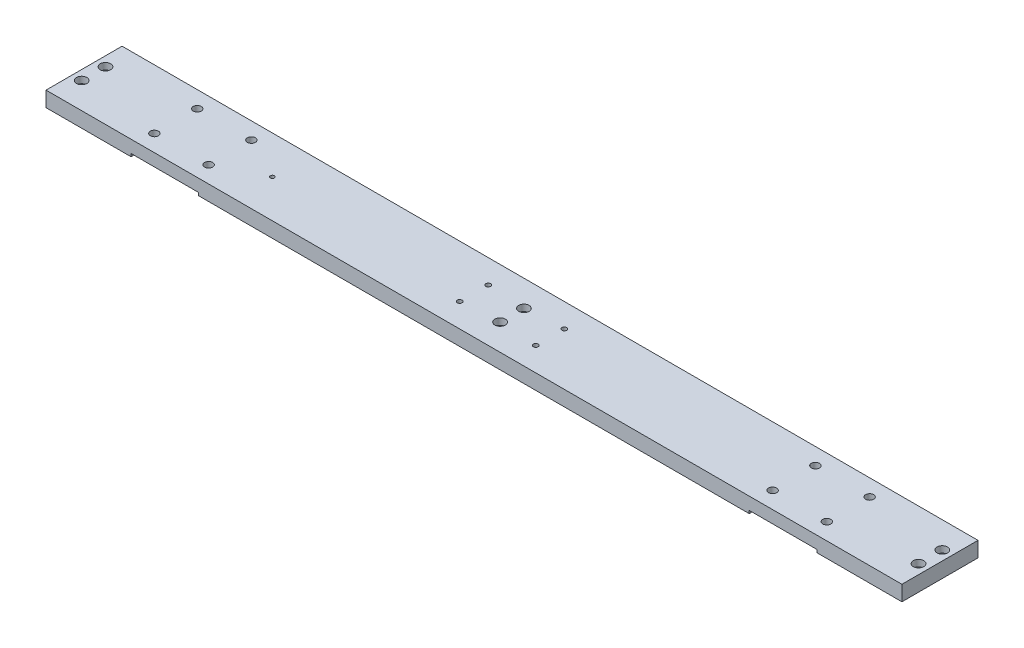
SolidWorks part; units mm, degrees
ref_plane "前视基准面" through (0, 0, 0) normal (0, 0, 1) x (1, 0, 0)
ref_plane "上视基准面" through (0, 0, 0) normal (0, 1, 0) x (1, 0, 0)
ref_plane "右视基准面" through (0, 0, 0) normal (1, 0, 0) x (0, 0, -1)
sketch "草图1" plane through (0, 0, 0) normal (0, 1, 0) x (1, 0, 0)
  line L1 (-450, 40) -> (450, 40)
  line L2 (-450, 40) -> (-450, -40)
  line L3 (-450, -40) -> (450, -40)
  line L4 (450, 40) -> (450, -40)
  line L5 (-450, 40) -> (450, -40) construction
  line L6 (-450, -40) -> (450, 40) construction
  point P0 (0, 0)
  dimension "D1" = 900
  dimension "D2" = 80
extrude "凸台-拉伸1" add sketch "草图1" along normal blind 16
sketch "草图2" plane through (0, 0, 0) normal (0, -1, 0) x (1, 0, 0)
  line L0 (-450, 40) -> (450, 40) construction
  line L1 (-360.549, 40) -> (-289.451, 40)
  line L2 (-360.549, 40) -> (-360.549, -40)
  line L3 (-360.549, -40) -> (-289.451, -40)
  line L4 (-289.451, 40) -> (-289.451, -40)
  line L5 (450, -40) -> (-450, -40) construction
  line L6 (0, 0) -> (0, 177.7451) construction
  line L7 (289.451, 40) -> (360.549, 40)
  line L8 (289.451, 40) -> (289.451, -40)
  line L9 (289.451, -40) -> (360.549, -40)
  line L10 (360.549, 40) -> (360.549, -40)
  dimension "D1" = 71.0981
  dimension "D2" = 650
extrude "切除-拉伸1" cut sketch "草图2" against normal blind 3
hole_wizard "Ø8.5 (8.5) 直径孔1" positions "草图3" profile "草图4" hole size "Ø8.5" standard "GB" end condition through all
sketch "草图3" plane through (0, 16, 0) normal (0, 1, 0) x (1, 0, 0)
  line L0 (0, 0) -> (-342.1751, 0) construction
  line L3 (-360.549, 40) -> (-289.451, 40) construction
  line L5 (-325, 40) -> (-325, 23.2164) construction
  point P0 (-353.5, 22.5)
  point P2 (-296.5, 22.5)
  point P4 (-353.5, -22.5)
  point P6 (-296.5, -22.5)
  dimension "D1" = 57
  dimension "D2" = 45
sketch "草图4" plane through (-353.5, 16, -22.5) normal (1, 0, 0) x (0, 0, 1)
  line L0 (0, 0) -> (0, 16)
  line L1 (0, 16) -> (4.25, 16)
  line L2 (4.25, 16) -> (4.25, 0)
  line L5 (4.25, 0) -> (0, 0)
  line L11 (0, -6.35) -> (0, 107.95) construction
  dimension "通孔孔直径" = 8.5
  dimension "通孔孔深度" = 16
mirror "镜向1" about plane through (0, 0, 0) normal (1, 0, 0) of "Ø8.5 (8.5) 直径孔1"
hole_wizard "M6 螺纹孔1" positions "草图5" profile "草图6" tap size "M6" standard "GB" end condition through all
sketch "草图5" plane through (0, 16, 0) normal (0, 1, 0) x (1, 0, 0)
  line L0 (0, 138.7998) -> (0, 0) construction
  line L1 (0, 0) -> (132.7322, 0) construction
  point P0 (-40, 15)
  point P2 (40, 15)
  point P4 (-40, -15)
  point P6 (40, -15)
  dimension "D1" = 80
  dimension "D2" = 30
sketch "草图6" plane through (-40, 16, -15) normal (1, 0, 0) x (0, 0, 1)
  line L0 (0, 0) -> (0, 16)
  line L1 (0, 16) -> (2.5, 16)
  line L2 (2.5, 16) -> (2.5, 0)
  line L5 (2.5, 0) -> (0, 0)
  line L11 (0, -6.35) -> (0, 107.95) construction
  dimension "通孔螺纹孔钻头直径" = 5
  dimension "通孔螺纹孔钻头深度" = 16
cosmetic thread "孔螺蚊线1" parameters "D2"=6
cosmetic thread "孔螺蚊线2" parameters "D2"=6
cosmetic thread "孔螺蚊线3" parameters "D2"=6
cosmetic thread "孔螺蚊线4" parameters "D2"=6
hole_wizard "打孔尺寸(%根据)内六角圆柱头螺钉的类型1" positions "草图7" profile "草图8" counterbore size "M6" standard "GB" end condition through all
sketch "草图7" plane through (0, 16, 0) normal (0, 1, 0) x (1, 0, 0)
  line L0 (-450, 0) -> (-385.8695, 0) construction
  line L1 (-450, 40) -> (-450, -40) construction
  point P0 (-440, 12.5)
  point P2 (-440, -12.5)
  dimension "D1" = 25
  dimension "D2" = 10
sketch "草图8" plane through (-440, 16, -12.5) normal (1, 0, 0) x (0, 0, 1)
  line L0 (0, 0) -> (0, 16)
  line L1 (0, 16) -> (3.3, 16)
  line L3 (3.3, 16) -> (3.3, 6.8)
  line L4 (3.3, 6.8) -> (5.5, 6.8)
  line L5 (5.5, 6.8) -> (5.5, 0)
  line L7 (5.5, 0) -> (0, 0)
  line L11 (0, -6.35) -> (0, 107.95) construction
  dimension "通孔孔直径" = 6.6
  dimension "通孔孔深度" = 16
  dimension "柱形沉头孔直径" = 11
  dimension "柱形沉头孔深度" = 6.8
pattern_linear "阵列(线性)1" count 3 spacing 440 along (1, 0, 0) of "打孔尺寸(%根据)内六角圆柱头螺钉的类型1"
hole_wizard "M5 螺纹孔1" positions "草图9" profile "草图10" tap size "M5" standard "GB" end condition through all
sketch "草图9" plane through (0, 16, 0) normal (0, 1, 0) x (1, 0, 0)
  line L0 (-450, 0) -> (-228.1839, 0) construction
  line L1 (-450, 40) -> (-450, -40) construction
  point P0 (-252, 0)
  dimension "D1" = 198
sketch "草图10" plane through (-252, 16, 0) normal (1, 0, 0) x (0, 0, 1)
  line L0 (0, 0) -> (0, 16)
  line L1 (0, 16) -> (2.1, 16)
  line L2 (2.1, 16) -> (2.1, 0)
  line L5 (2.1, 0) -> (0, 0)
  line L11 (0, -6.35) -> (0, 107.95) construction
  dimension "通孔螺纹孔钻头直径" = 4.2
  dimension "通孔螺纹孔钻头深度" = 16
cosmetic thread "孔螺蚊线5" parameters "D2"=5
